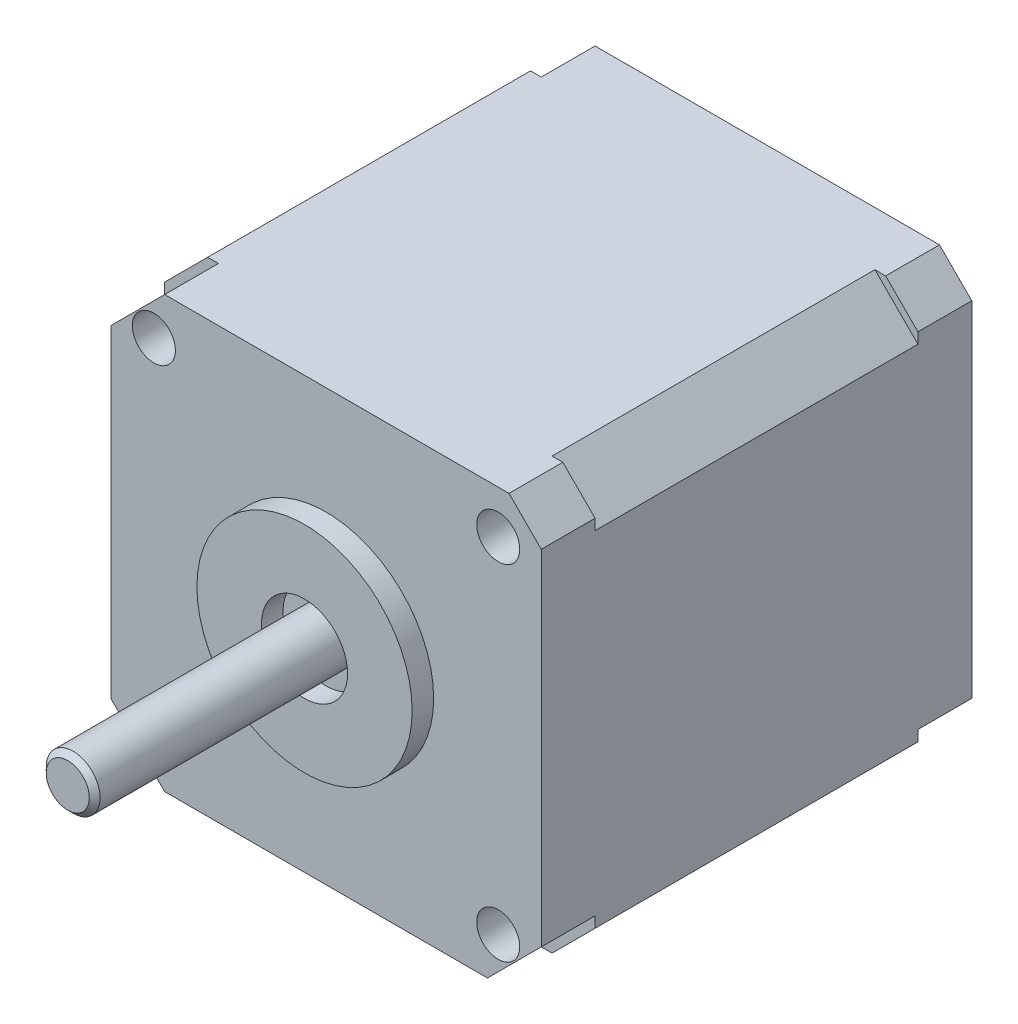
SolidWorks part; units mm, degrees
material "Nickel"
ref_plane "Front Plane" through (0, 0, 0) normal (0, 0, 1) x (1, 0, 0)
ref_plane "Top Plane" through (0, 0, 0) normal (0, 1, 0) x (1, 0, 0)
ref_plane "Right Plane" through (0, 0, 0) normal (1, 0, 0) x (0, 0, -1)
sketch "Sketch1" plane through (0, 0, 0) normal (0, 0, 1) x (1, 0, 0)
  line L1 (20, -20) -> (-20, -20)
  line L2 (20, -20) -> (20, 20)
  line L3 (20, 20) -> (-20, 20)
  line L4 (-20, -20) -> (-20, 20)
  line L5 (20, -20) -> (-20, 20) construction
  line L6 (20, 20) -> (-20, -20) construction
  point P0 (0, 0)
  dimension "D1" = 40
  dimension "D2" = 40
extrude "Boss-Extrude1" add sketch "Sketch1" along normal mid plane 30
chamfer "Chamfer1" distance 4 angle 45 4 edges at (-20, -20, 0) (20, -20, 0) (-20, 20, 0) (20, 20, 0)
sketch "Sketch3" plane through (0, 0, 15) normal (0, 0, 1) x (1, 0, 0)
  line L0 (16, 20) -> (-16, 20) construction
  line L1 (15, -20) -> (-15, -20)
  line L2 (20, -15) -> (20, 17)
  line L3 (17, 20) -> (-15, 20)
  line L4 (-20, -15) -> (-20, 15)
  line L5 (20, -20) -> (-20, 20) construction
  line L6 (20, 20) -> (-20, -20) construction
  line L7 (-20, 16) -> (-20, -16) construction
  line L8 (-15, 20) -> (-20, 15)
  line L9 (20, 17) -> (17, 20)
  line L10 (20, -15) -> (15, -20)
  line L11 (-15, -20) -> (-20, -15)
  point P0 (0, 0)
  dimension "D1" = 5
  dimension "D2" = 45
  dimension "D3" = 3
  dimension "D4" = 45
  dimension "D5" = 5
  dimension "D6" = 45
  dimension "D7" = 5
  dimension "D8" = 45
extrude "Boss-Extrude2" add sketch "Sketch3" along normal blind 5
mirror "Mirror1" about plane through (0, 0, 0) normal (0, 0, 1) of "Boss-Extrude2"
sketch "Sketch4" plane through (0, 0, 20) normal (0, 0, 1) x (1, 0, 0)
  circle A0 centre (0, 0) radius 10
  dimension "D1" = 20
extrude "Boss-Extrude3" add sketch "Sketch4" along normal blind 2
sketch "Sketch5" plane through (0, 0, 22) normal (0, 0, 1) x (1, 0, 0)
  circle A0 centre (0, 0) radius 2.5
  dimension "D1" = 5
extrude "Boss-Extrude4" add sketch "Sketch5" along normal blind 22
sketch "Sketch6" plane through (0, 0, 22) normal (0, 0, 1) x (1, 0, 0)
  circle A0 centre (0, 0) radius 4
  circle A1 centre (0, 0) radius 2.5
  circle A2 centre (0, 0) radius 2.5
  dimension "D2" = 8
  dimension "D1" = 0
extrude "Cut-Extrude1" cut sketch "Sketch6" against normal blind 2
chamfer "Chamfer2" distance 0.5 angle 45 1 edges at (2.5, 0, 44)
sketch "Sketch7" plane through (0, 0, 20) normal (0, 0, 1) x (1, 0, 0)
  circle A0 centre (16, 16) radius 2
  circle A1 centre (16, -16) radius 2
  circle A2 centre (-16, -16) radius 2
  circle A3 centre (-16, 16) radius 2
  point P12 (0, 0)
  dimension "D1" = 4
  dimension "D2" = 16
  dimension "D3" = 16
  dimension "D4" = 4
extrude "Cut-Extrude2" cut sketch "Sketch7" against normal through all
